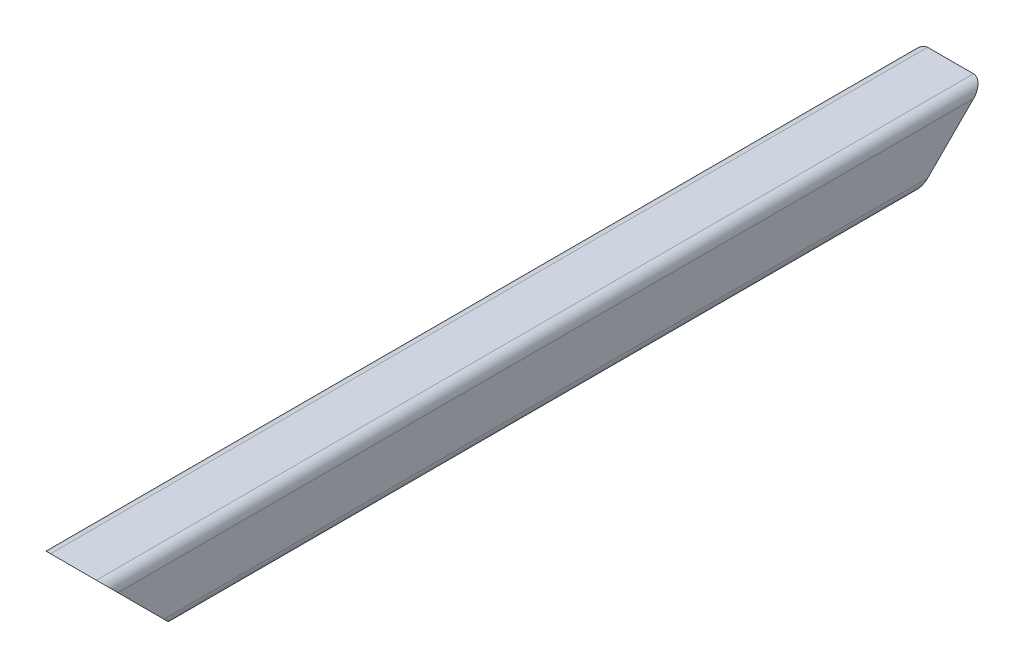
SolidWorks part; units mm, degrees
material "AISI 1045 钢，冷拔"
ref_plane "Front Plane" through (0, 0, 0) normal (0, 0, 1) x (1, 0, 0)
ref_plane "Top Plane" through (0, 0, 0) normal (0, 1, 0) x (1, 0, 0)
ref_plane "Right Plane" through (0, 0, 0) normal (1, 0, 0) x (0, 0, -1)
sketch "Sketch1" plane through (0, 0, 0) normal (0, 0, 1) x (1, 0, 0)
  line L0 (-21.0947, 0) -> (28.2454, 0) construction
  line L1 (0, 28.305) -> (0, -28.2454) construction
  line L2 (-17, 21) -> (17, 21)
  line L3 (-17, -25) -> (17, -25)
  line L4 (-25, -17) -> (-25, 17)
  line L5 (-17, 25) -> (17, 25)
  line L6 (25, -17) -> (25, 17)
  line L7 (-25, -25) -> (25, 25) construction
  line L8 (-25, 25) -> (25, -25) construction
  line L9 (21, -17) -> (21, 17)
  line L10 (-17, -21) -> (17, -21)
  line L11 (-21, -17) -> (-21, 17)
  arc A0 (17, -25) -> (25, -17) centre (17, -17) ccw
  arc A1 (-17, -25) -> (-25, -17) centre (-17, -17) cw
  arc A2 (17, 25) -> (25, 17) centre (17, 17) cw
  arc A3 (-25, 17) -> (-17, 25) centre (-17, 17) cw
  arc A4 (-21, 17) -> (-17, 21) centre (-17, 17) cw
  arc A5 (17, 21) -> (21, 17) centre (17, 17) cw
  arc A6 (17, -21) -> (21, -17) centre (17, -17) ccw
  arc A7 (-17, -21) -> (-21, -17) centre (-17, -17) cw
  point P5 (0, 0)
  dimension "D3" = 8
  dimension "D1" = 50
  dimension "D2" = 50
  dimension "D4" = 4
extrude "Boss-Extrude1" add sketch "Sketch1" along normal mid plane 650
sketch "Sketch2" plane through (-25, 0, 0) normal (-1, 0, 0) x (0, 0, 1)
  line L0 (-325, 25) -> (-275, -25)
  line L1 (325, -25) -> (-325, -25) construction
  line L2 (-275, -25) -> (-325, -25)
  line L3 (-325, -25) -> (-325, 25)
  dimension "D1" = 45
extrude "Cut-Extrude1" cut sketch "Sketch2" against normal through all
mirror "Mirror1" about plane through (0, 0, 0) normal (0, 0, 1) of "Cut-Extrude1"
